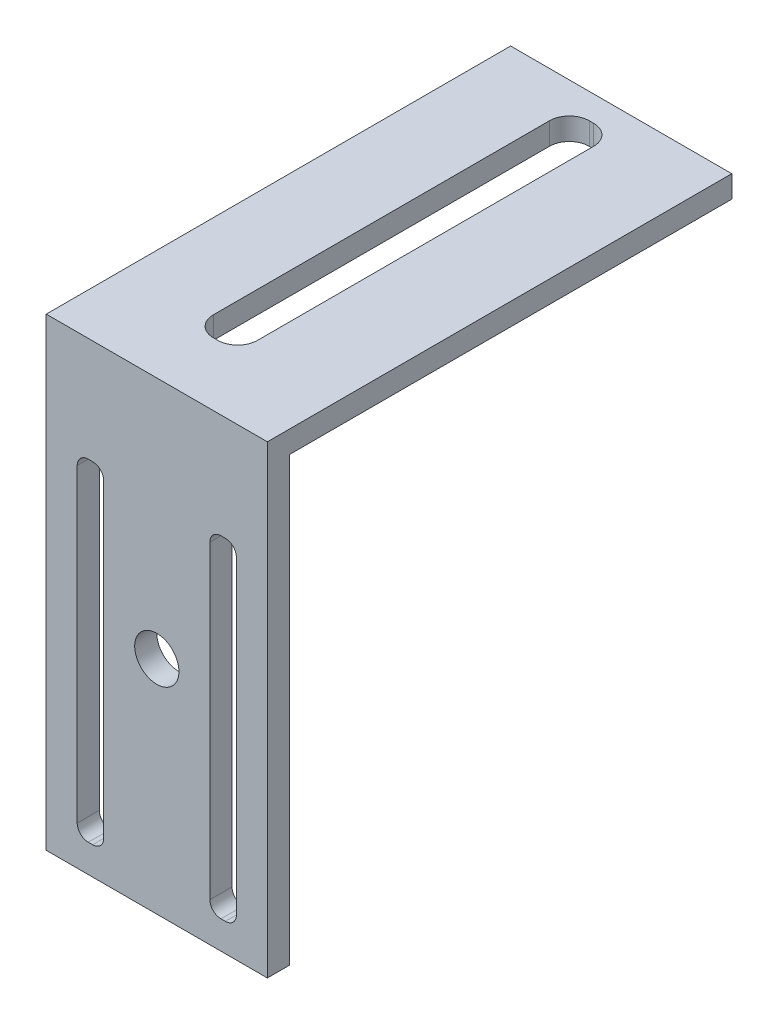
SolidWorks part; units mm, degrees
ref_plane "Front Plane" through (0, 0, 0) normal (0, 0, 1) x (1, 0, 0)
ref_plane "Top Plane" through (0, 0, 0) normal (0, 1, 0) x (1, 0, 0)
ref_plane "Right Plane" through (0, 0, 0) normal (1, 0, 0) x (0, 0, -1)
sketch "Sketch1" plane through (0, 0, 0) normal (0, 0, 1) x (1, 0, 0)
  line L1 (25, -50) -> (-25, -50)
  line L2 (25, -50) -> (25, 50)
  line L3 (25, 50) -> (-25, 50)
  line L4 (-25, -50) -> (-25, 50)
  line L5 (25, -50) -> (-25, 50) construction
  line L6 (25, 50) -> (-25, -50) construction
  point P0 (0, 0)
  dimension "D1" = 100
  dimension "D2" = 50
extrude "Boss-Extrude1" add sketch "Sketch1" along normal blind 5
sketch "Sketch2" plane through (0, 0, 5) normal (0, 0, 1) x (1, 0, 0)
  line L0 (0, 32.1879) -> (0, -24.1157) construction
  line L1 (-15, 24.3175) -> (-15, -24.1157) construction
  line L2 (15, 24.3175) -> (15, -24.1157) construction
  line L4 (-14.5, -43.6551) -> (-15.5, -43.6551)
  line L5 (-12, -41.1551) -> (-12, 28.8449)
  line L6 (-14.5, 31.3449) -> (-15.5, 31.3449)
  line L7 (-18, -41.1551) -> (-18, 28.8449)
  line L8 (-12, -43.6551) -> (-18, 31.3449) construction
  line L9 (-12, 31.3449) -> (-18, -43.6551) construction
  line L10 (15.5, -43.6551) -> (14.5, -43.6551)
  line L11 (18, -41.1551) -> (18, 28.8449)
  line L12 (15.5, 31.3449) -> (14.5, 31.3449)
  line L13 (12, -41.1551) -> (12, 28.8449)
  line L14 (18, -43.6551) -> (12, 31.3449) construction
  line L15 (18, 31.3449) -> (12, -43.6551) construction
  arc A0 (14.5, 31.3449) -> (12, 28.8449) centre (14.5, 28.8449) ccw
  arc A1 (18, 28.8449) -> (15.5, 31.3449) centre (15.5, 28.8449) ccw
  arc A2 (14.5, -43.6551) -> (12, -41.1551) centre (14.5, -41.1551) cw
  arc A3 (15.5, -43.6551) -> (18, -41.1551) centre (15.5, -41.1551) ccw
  arc A4 (-15.5, -43.6551) -> (-18, -41.1551) centre (-15.5, -41.1551) cw
  arc A5 (-14.5, -43.6551) -> (-12, -41.1551) centre (-14.5, -41.1551) ccw
  arc A6 (-12, 28.8449) -> (-14.5, 31.3449) centre (-14.5, 28.8449) ccw
  arc A7 (-15.5, 31.3449) -> (-18, 28.8449) centre (-15.5, 28.8449) ccw
  point P7 (-15, -6.1551)
  point P12 (15, -6.1551)
  dimension "D7" = 2.5
  dimension "D1" = 15
  dimension "D2" = 15
  dimension "D3" = 6
  dimension "D4" = 6
  dimension "D5" = 75
  dimension "D6" = 75
extrude "Cut-Extrude1" cut sketch "Sketch2" against normal blind 10
sketch "Sketch3" plane through (0, 0, 5) normal (0, 0, 1) x (1, 0, 0)
  circle A0 centre (0, 0) radius 5
  dimension "D1" = 10
extrude "Cut-Extrude2" cut sketch "Sketch3" against normal blind 10
sketch "Sketch4" plane through (0, 0, 0) normal (0, 0, -1) x (-1, 0, 0)
  line L0 (-25, 50) -> (-25, 55)
  line L1 (25, 50) -> (25, 55)
  line L2 (25, 55) -> (-25, 55)
  line L3 (25, 50) -> (-25, 50)
  dimension "D1" = 5
extrude "Boss-Extrude2" add sketch "Sketch4" along normal blind 100 and the other way blind 5
sketch "Sketch5" plane through (0, 50, 0) normal (0, -1, 0) x (1, 0, 0)
  line L1 (-0.474, -94.2529) -> (-1.474, -94.2529)
  line L2 (4.026, -89.7529) -> (4.026, -13.7529)
  line L3 (-0.474, -9.2529) -> (-1.474, -9.2529)
  line L4 (-5.974, -89.7529) -> (-5.974, -13.7529)
  line L5 (4.026, -94.2529) -> (-5.974, -9.2529) construction
  line L6 (4.026, -9.2529) -> (-5.974, -94.2529) construction
  arc A0 (-1.474, -94.2529) -> (-5.974, -89.7529) centre (-1.474, -89.7529) cw
  arc A1 (-0.474, -94.2529) -> (4.026, -89.7529) centre (-0.474, -89.7529) ccw
  arc A2 (4.026, -13.7529) -> (-0.474, -9.2529) centre (-0.474, -13.7529) ccw
  arc A3 (-1.474, -9.2529) -> (-5.974, -13.7529) centre (-1.474, -13.7529) ccw
  point P0 (-0.974, -51.7529)
  dimension "D3" = 4.5
  dimension "D1" = 10
  dimension "D2" = 85
extrude "Cut-Extrude3" cut sketch "Sketch5" against normal blind 80
